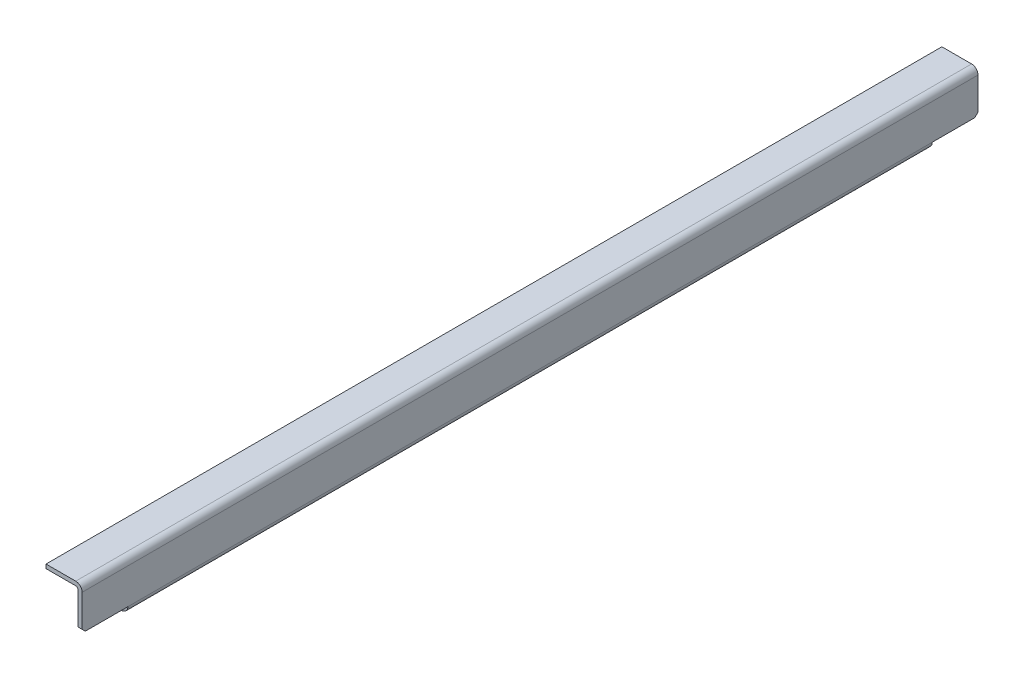
SolidWorks part; units mm, degrees
material "1023 碳钢板 (SS)"
ref_plane "Front Plane" through (0, 0, 0) normal (0, 0, 1) x (1, 0, 0)
ref_plane "Top Plane" through (0, 0, 0) normal (0, 1, 0) x (1, 0, 0)
ref_plane "Right Plane" through (0, 0, 0) normal (1, 0, 0) x (0, 0, -1)
sketch "Sketch1" plane through (0, 0, 0) normal (0, 0, 1) x (1, 0, 0)
  line L0 (0, 0) -> (37, 0)
  line L1 (45, -8) -> (45, -52)
  line L2 (37, -60) -> (0, -60)
  line L3 (0, -5) -> (37, -5)
  line L4 (40, -8) -> (40, -52)
  line L5 (37, -55) -> (0, -55)
  line L6 (0, 0) -> (0, -5)
  line L7 (0, -55) -> (0, -60)
  arc A0 (45, -52) -> (37, -60) centre (37, -52) cw
  arc A1 (37, 0) -> (45, -8) centre (37, -8) cw
  arc A2 (37, -5) -> (40, -8) centre (37, -8) cw
  arc A3 (40, -52) -> (37, -55) centre (37, -52) cw
  point P7 (45, -60)
  point P10 (45, 0)
  dimension "D4" = 8
  dimension "D1" = 45
  dimension "D2" = 60
  dimension "D3" = 45
  dimension "D5" = 5
extrude "Boss-Extrude1" add sketch "Sketch1" along normal blind 1116 contours L7 L2 A0 L1 A1 L0 L6 L3 A2 L4 A3 L5
sketch "Sketch2" plane through (0, 0, 0) normal (-1, 0, 0) x (0, 0, 1)
  line L0 (1116, -60) -> (0, -60) construction
  line L1 (1059, -52) -> (1151.4751, -52)
  line L2 (1059, -52) -> (1059, -90.6467)
  line L3 (1059, -90.6467) -> (1151.4751, -90.6467)
  line L4 (1151.4751, -52) -> (1151.4751, -90.6467)
  line L5 (1059, -52) -> (1151.4751, -90.6467) construction
  line L6 (1059, -90.6467) -> (1151.4751, -52) construction
  line L7 (1116, -8) -> (1116, -52) construction
  line L8 (0, -8) -> (0, -52) construction
  line L9 (57, -96.8575) -> (-33.3973, -96.8575)
  line L10 (57, -96.8575) -> (57, -52)
  line L11 (57, -52) -> (-33.3973, -52)
  line L12 (-33.3973, -96.8575) -> (-33.3973, -52)
  line L13 (57, -96.8575) -> (-33.3973, -52) construction
  line L14 (57, -52) -> (-33.3973, -96.8575) construction
  point P0 (1105.2376, -71.3233)
  point P9 (11.8014, -74.4287)
  dimension "D1" = 8
  dimension "D2" = 57
  dimension "D3" = 57
  dimension "D4" = 8
extrude "Cut-Extrude1" cut sketch "Sketch2" against normal blind 1116
sketch "Sketch3" plane through (0, -55, 0) normal (0, 1, 0) x (1, 0, 0)
  line L1 (0, 0) -> (37, 0) construction
  line L2 (0, -1116) -> (0, 0) construction
  circle A2 centre (12.5, -92) radius 4
  dimension "D1" = 92
  dimension "D3" = 12.5
  dimension "D6" = 8
extrude "Cut-Extrude2" cut sketch "Sketch3" against normal blind 1116
hole_wizard "M10 Tapped Hole1" positions "Sketch4" profile "Sketch5" tap size "M10" standard "ISO"
sketch "Sketch4" plane through (0, -55, 0) normal (0, 1, 0) x (1, 0, 0)
  point P0 (12.5, -92)
sketch "Sketch5" plane through (12.5, -55, 92) normal (1, 0, 0) x (0, 0, 1)
  line L0 (0, 0) -> (0, 27.0537)
  line L1 (0, 27.0537) -> (4.25, 24.5)
  line L2 (4.25, 24.5) -> (4.25, 0)
  line L5 (4.25, 0) -> (0, 0)
  line L10 (0, 27.0537) -> (-4.25, 24.5) construction
  line L11 (0, -6.35) -> (0, 107.95) construction
  dimension "螺纹孔钻头直径" = 8.5
  dimension "螺纹孔钻头深度" = 24.5
  dimension "导头角度" = 118
cosmetic thread "Hole Thread Line1" parameters "D1"=20, "D2"=10
chamfer "Chamfer1" distance 4 angle 45 2 edges at (42.5, -52, 0) (42.5, -52, 1116)
